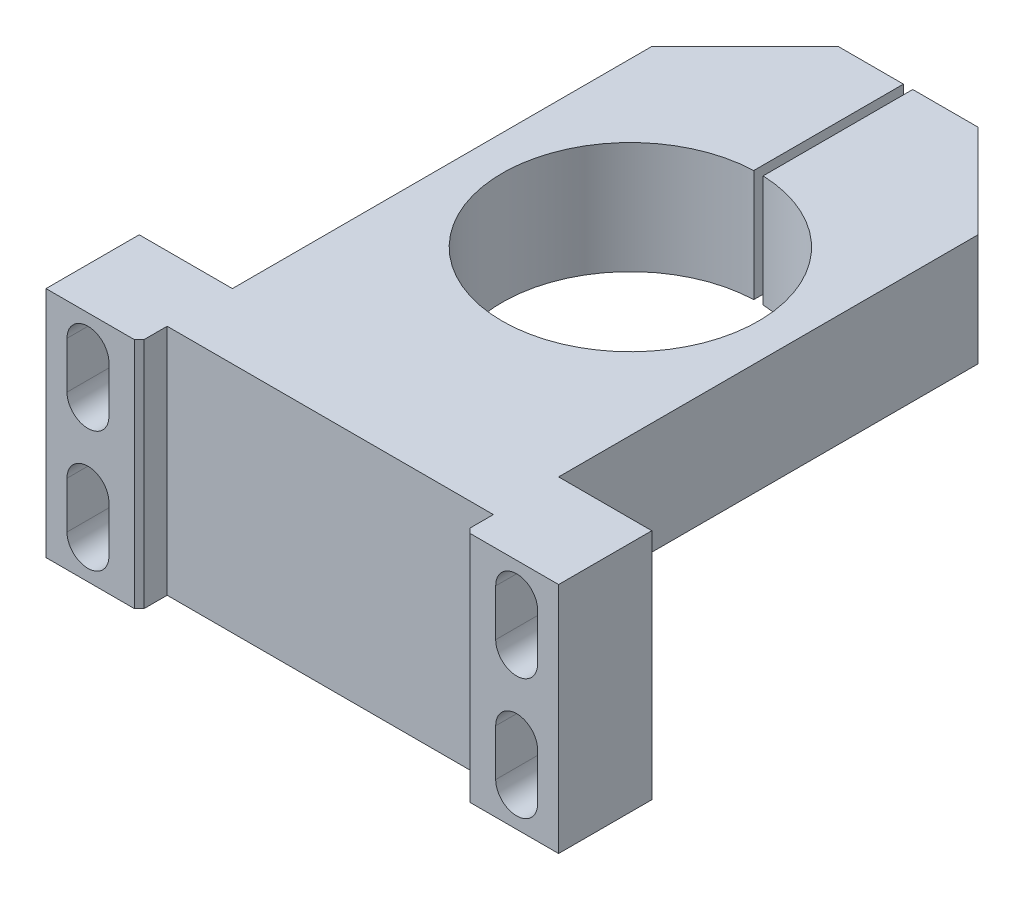
from build123d import *

# Parameters (mm, degrees)
SKETCH1_W           = 35
SKETCH1_H           = 65
SKETCH1_R           = 13.75
BOSS_EXTRUDE1_DEPTH = 12
CHAMFER1_SIZE       = 10
SKETCH2_W           = 55
SKETCH2_H           = 10
BOSS_EXTRUDE2_DEPTH = 25
SKETCH3_W           = 35
SKETCH3_H           = 6
CUT_EXTRUDE1_DEPTH  = 52.188768299
CUT_EXTRUDE2_DEPTH  = 13.5
CHAMFER2_SIZE       = 0.5
SKETCH5_W           = 1
SKETCH5_H           = 37.783958766
CUT_EXTRUDE3_DEPTH  = 52.188768299
SKETCH6_R           = 5
CUT_EXTRUDE4_DEPTH  = 10
SKETCH7_R           = 2.25
CUT_EXTRUDE5_DEPTH  = 7
M4_TAPPED_HOLE1_D   = 3.3


with BuildPart() as part:
    # Sketch1 → Boss-Extrude1 (new body)
    with BuildSketch(Plane(origin=(0, 0, 0), x_dir=(1, 0, 0), z_dir=(0, 1, 0))):
        with Locations((0, -2.7)):
            Rectangle(SKETCH1_W, SKETCH1_H)
        with Locations(Location((0, 0, 0), (0, 0, 270))):
            Circle(SKETCH1_R, mode=Mode.SUBTRACT)
    extrude(amount=BOSS_EXTRUDE1_DEPTH)

    # Chamfer1
    chamfer1_edges = [part.edges().sort_by_distance(p)[0] for p in [
        (-17.5, 6, -29.8),
        (17.5, 6, -29.8),
    ]]
    chamfer(chamfer1_edges, length=CHAMFER1_SIZE)

    # Sketch2 → Boss-Extrude2 (add)
    with BuildSketch(Plane(origin=(0, 12, 0), x_dir=(1, 0, 0), z_dir=(0, 1, 0))):
        with Locations((0, -30.2)):
            Rectangle(SKETCH2_W, SKETCH2_H)
    extrude(amount=-BOSS_EXTRUDE2_DEPTH)

    # Sketch3 → Cut-Extrude1 (cut, through all)
    with BuildSketch(Plane.XZ.offset(13)):
        with Locations((0, 35.2)):
            Rectangle(SKETCH3_W, SKETCH3_H)
    extrude(amount=-CUT_EXTRUDE1_DEPTH, mode=Mode.SUBTRACT)

    # Sketch4 → Cut-Extrude2 (cut)
    with BuildSketch(Plane(origin=(0, 0, 25.2), x_dir=(-1, 0, 0), z_dir=(0, 0, -1))):
        with BuildLine():
            Line((-20.75, 8.5), (-20.75, 3.5))
            ThreePointArc((-20.75, 3.5), (-23, 1.25), (-25.25, 3.5))
            Line((-25.25, 3.5), (-25.25, 8.5))
            ThreePointArc((-25.25, 8.5), (-23, 10.75), (-20.75, 8.5))
        make_face()
        with BuildLine():
            Line((20.75, 8.5), (20.75, 3.5))
            ThreePointArc((20.75, 3.5), (23, 1.25), (25.25, 3.5))
            Line((25.25, 3.5), (25.25, 8.5))
            ThreePointArc((25.25, 8.5), (23, 10.75), (20.75, 8.5))
        make_face()
        with BuildLine():
            Line((20.75, -9.5), (20.75, -4.5))
            ThreePointArc((20.75, -4.5), (23, -2.25), (25.25, -4.5))
            Line((25.25, -4.5), (25.25, -9.5))
            ThreePointArc((25.25, -9.5), (23, -11.75), (20.75, -9.5))
        make_face()
        with BuildLine():
            Line((-20.75, -9.5), (-20.75, -4.5))
            ThreePointArc((-20.75, -4.5), (-23, -2.25), (-25.25, -4.5))
            Line((-25.25, -4.5), (-25.25, -9.5))
            ThreePointArc((-25.25, -9.5), (-23, -11.75), (-20.75, -9.5))
        make_face()
    extrude(amount=-CUT_EXTRUDE2_DEPTH, mode=Mode.SUBTRACT)

    # Chamfer2
    chamfer2_edges = [part.edges().sort_by_distance(p)[0] for p in [
        (17.5, -0.5, 35.2),
        (-17.5, -0.5, 35.2),
    ]]
    chamfer(chamfer2_edges, length=CHAMFER2_SIZE)

    # Sketch5 → Cut-Extrude3 (cut, through all)
    with BuildSketch(Plane(origin=(0, 12, 0), x_dir=(1, 0, 0), z_dir=(0, 1, 0))):
        with Locations((0, 29.8)):
            Rectangle(SKETCH5_W, SKETCH5_H)
    extrude(amount=-CUT_EXTRUDE3_DEPTH, mode=Mode.SUBTRACT)

    # Sketch6 → Cut-Extrude4 (cut)
    with BuildSketch(Plane.ZY.offset(17.5)):
        with Locations((-21.8, 6)):
            Circle(SKETCH6_R)
    extrude(amount=-CUT_EXTRUDE4_DEPTH, mode=Mode.SUBTRACT)

    # Sketch7 → Cut-Extrude5 (cut)
    with BuildSketch(Plane.ZY.offset(7.5)):
        with Locations((-21.8, 6)):
            Circle(SKETCH7_R)
    extrude(amount=-CUT_EXTRUDE5_DEPTH, mode=Mode.SUBTRACT)

    # M4 Tapped Hole1 (through all)
    with Locations(Plane.ZY.offset(-0.5)):
        with Locations((-21.8, 6)):
            Hole(M4_TAPPED_HOLE1_D / 2)


solid = part.part
